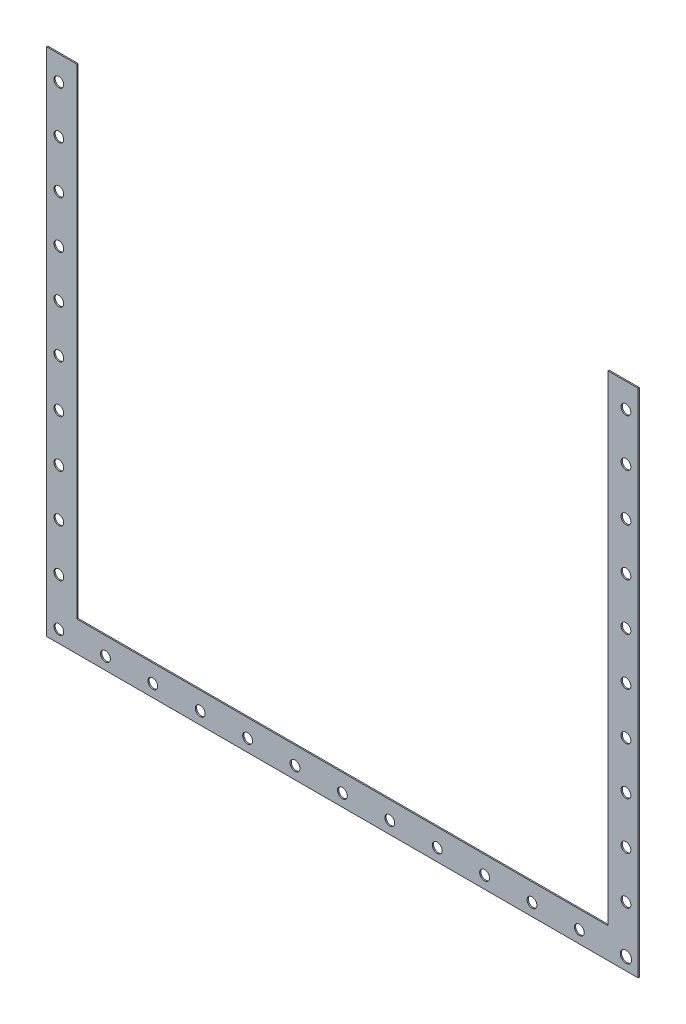
from build123d import *

# Parameters (mm, degrees)
SKETCH1_R           = 12
SKETCH1_R_2         = 13.848900056
BOSS_EXTRUDE1_DEPTH = 3


with BuildPart() as part:
    # Sketch1 → Boss-Extrude1 (new body)
    # profile 1 of 2: a face of its own
    with BuildSketch(Plane.XY):
        with BuildLine():
            Line((7.821297611, 64.305720246), (-66.178702389, 64.305720246))
            Line((-66.178702389, 64.305720246), (-66.178702389, -1185.694279754))
            Line((-66.178702389, -1185.694279754), (657.821297611, -1185.694279754))
            Line((657.821297611, -1185.694279754), (657.821297611, -1167.694279754))
            ThreePointArc((657.821297611, -1167.694279754), (645.821297611, -1155.694279754), (657.821297611, -1143.694279754))
            Line((657.821297611, -1143.694279754), (657.821297611, -1111.694279754))
            Line((657.821297611, -1111.694279754), (7.821297611, -1111.694279754))
            Line((7.821297611, -1111.694279754), (7.821297611, 64.305720246))
        make_face()
        with Locations((-36.178702389, -1155.694279754)):
            Circle(SKETCH1_R, mode=Mode.SUBTRACT)
        with Locations((77.821297611, -1155.694279754)):
            Circle(SKETCH1_R, mode=Mode.SUBTRACT)
        with Locations((-36.178702389, -1039.694279754)):
            Circle(SKETCH1_R, mode=Mode.SUBTRACT)
        with Locations((193.821297611, -1155.694279754)):
            Circle(SKETCH1_R, mode=Mode.SUBTRACT)
        with Locations((-36.178702389, -923.694279754)):
            Circle(SKETCH1_R, mode=Mode.SUBTRACT)
        with Locations((309.821297611, -1155.694279754)):
            Circle(SKETCH1_R, mode=Mode.SUBTRACT)
        with Locations((425.821297611, -1155.694279754)):
            Circle(SKETCH1_R, mode=Mode.SUBTRACT)
        with Locations((541.821297611, -1155.694279754)):
            Circle(SKETCH1_R, mode=Mode.SUBTRACT)
        with Locations((-36.178702389, -807.694279754)):
            Circle(SKETCH1_R, mode=Mode.SUBTRACT)
        with Locations((-36.178702389, -691.694279754)):
            Circle(SKETCH1_R, mode=Mode.SUBTRACT)
        with Locations((-36.178702389, -575.694279754)):
            Circle(SKETCH1_R, mode=Mode.SUBTRACT)
        with Locations((-36.178702389, -459.694279754)):
            Circle(SKETCH1_R, mode=Mode.SUBTRACT)
        with Locations((-36.178702389, -343.694279754)):
            Circle(SKETCH1_R, mode=Mode.SUBTRACT)
        with Locations((-36.178702389, -227.694279754)):
            Circle(SKETCH1_R, mode=Mode.SUBTRACT)
        with Locations((-36.178702389, -111.694279754)):
            Circle(SKETCH1_R, mode=Mode.SUBTRACT)
        with Locations((-36.178702389, 4.305720246)):
            Circle(SKETCH1_R, mode=Mode.SUBTRACT)
    # profile 2 of 2: a face of its own
    with BuildSketch(Plane.XY):
        with BuildLine():
            Line((657.821297611, -1167.694279754), (657.821297611, -1185.694279754))
            Line((657.821297611, -1185.694279754), (1381.821297611, -1185.694279754))
            Line((1381.821297611, -1185.694279754), (1381.821297611, 64.305720246))
            Line((1381.821297611, 64.305720246), (1307.821297611, 64.305720246))
            Line((1307.821297611, 64.305720246), (1307.821297611, -1111.694279754))
            Line((1307.821297611, -1111.694279754), (657.821297611, -1111.694279754))
            Line((657.821297611, -1111.694279754), (657.821297611, -1143.694279754))
            ThreePointArc((657.821297611, -1143.694279754), (666.306578985, -1147.20899838), (669.821297611, -1155.694279754))
            ThreePointArc((669.821297611, -1155.694279754), (666.306578985, -1164.179561128), (657.821297611, -1167.694279754))
        make_face()
        with Locations((773.821297611, -1155.694279754)):
            Circle(SKETCH1_R, mode=Mode.SUBTRACT)
        with Locations((889.821297611, -1155.694279754)):
            Circle(SKETCH1_R, mode=Mode.SUBTRACT)
        with Locations((1005.821297611, -1155.694279754)):
            Circle(SKETCH1_R, mode=Mode.SUBTRACT)
        with Locations((1121.821297611, -1155.694279754)):
            Circle(SKETCH1_R, mode=Mode.SUBTRACT)
        with Locations((1237.821297611, -1155.694279754)):
            Circle(SKETCH1_R, mode=Mode.SUBTRACT)
        with Locations((1351.821297611, -1155.694279754)):
            Circle(SKETCH1_R_2, mode=Mode.SUBTRACT)
        with Locations((1351.821297611, -1039.694279754)):
            Circle(SKETCH1_R, mode=Mode.SUBTRACT)
        with Locations((1351.821297611, -923.694279754)):
            Circle(SKETCH1_R, mode=Mode.SUBTRACT)
        with Locations((1351.821297611, -807.694279754)):
            Circle(SKETCH1_R, mode=Mode.SUBTRACT)
        with Locations((1351.821297611, -691.694279754)):
            Circle(SKETCH1_R, mode=Mode.SUBTRACT)
        with Locations((1351.821297611, -575.694279754)):
            Circle(SKETCH1_R, mode=Mode.SUBTRACT)
        with Locations((1351.821297611, -459.694279754)):
            Circle(SKETCH1_R, mode=Mode.SUBTRACT)
        with Locations((1351.821297611, -343.694279754)):
            Circle(SKETCH1_R, mode=Mode.SUBTRACT)
        with Locations((1351.821297611, -227.694279754)):
            Circle(SKETCH1_R, mode=Mode.SUBTRACT)
        with Locations((1351.821297611, -111.694279754)):
            Circle(SKETCH1_R, mode=Mode.SUBTRACT)
        with Locations((1351.821297611, 4.305720246)):
            Circle(SKETCH1_R, mode=Mode.SUBTRACT)
    extrude(amount=BOSS_EXTRUDE1_DEPTH)


solid = part.part
